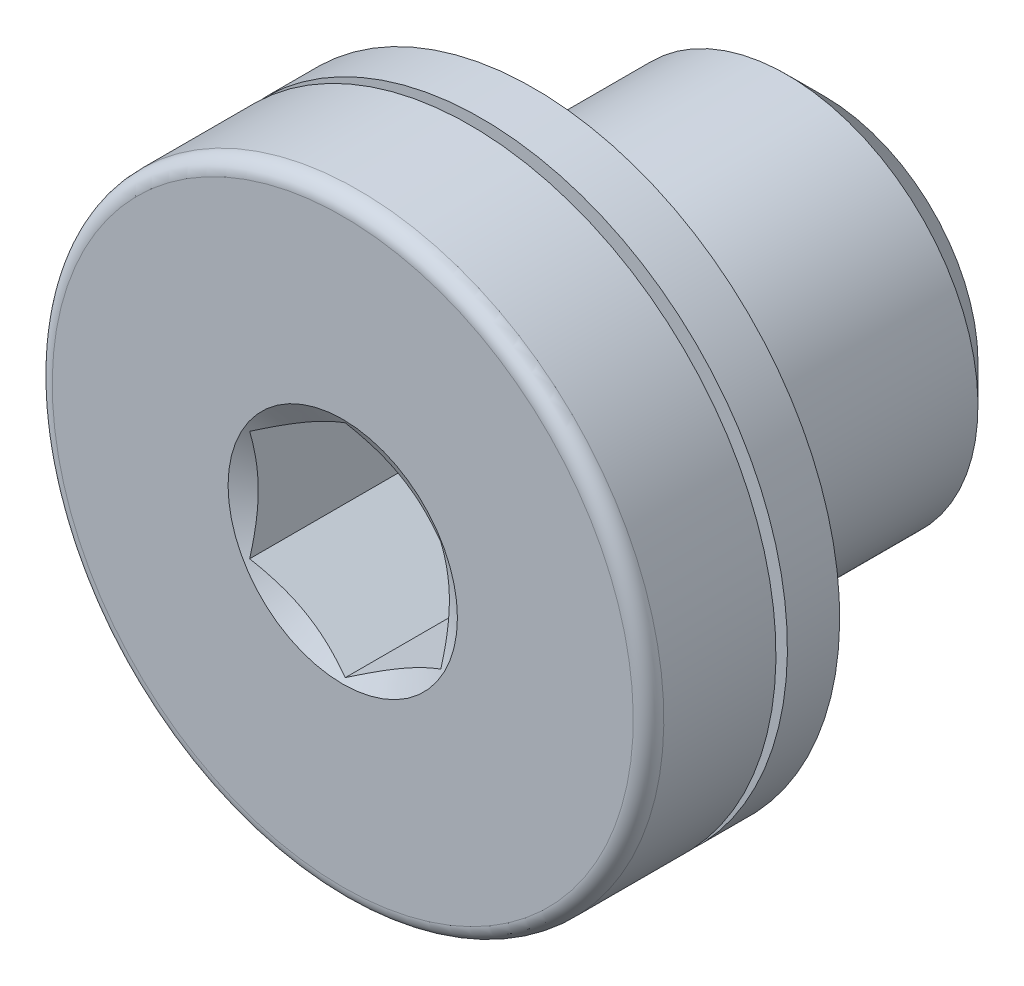
from build123d import *

# Parameters (mm, degrees)
CUT_EXTRUDE1_DEPTH = 2.5


with BuildPart() as part:
    # Sketch1 → Revolve1 (revolve)
    with BuildSketch(Plane(origin=(0, 0, 0), x_dir=(0, 0, -1), z_dir=(1, 0, 0)), mode=Mode.PRIVATE) as revolve1_sk:
        with BuildLine():
            Line((-1.633974596, 0), (-2.5, 1.5))
            Line((-2.5, 1.5), (-2.5, 3.8))
            ThreePointArc((-2.5, 3.8), (-2.441421356, 3.941421356), (-2.3, 4))
            Line((-2.3, 4), (-0.833333333, 4))
            Line((-0.833333333, 4), (-0.833333333, 3.6))
            Line((-0.833333333, 3.6), (-0.683333333, 3.6))
            Line((-0.683333333, 3.6), (-0.683333333, 4))
            Line((-0.683333333, 4), (0, 4))
            Line((0, 4), (0, 2.0095))
            Line((0, 2.0095), (0.4905, 2.5))
            Line((0.4905, 2.5), (3.3095, 2.5))
            Line((3.3095, 2.5), (3.8, 2.0095))
            Line((3.8, 2.0095), (3.8, 0))
            Line((3.8, 0), (-1.633974596, 0))
        make_face()
    revolve(revolve1_sk.sketch.rotate(Axis((0, 0, -3.8), (0, 0, 1)), 180), axis=Axis((0, 0, -3.8), (0, 0, 1)))

    # Sketch2 → Cut-Extrude1 (cut)
    with BuildSketch(Plane.XY.offset(2.5)):
        Polygon((-1.25, -0.721687836), (0, -1.443375673), (1.25, -0.721687836), (1.25, 0.721687836), (0, 1.443375673), (-1.25, 0.721687836), align=None)
    extrude(amount=-CUT_EXTRUDE1_DEPTH, mode=Mode.SUBTRACT)


solid = part.part
